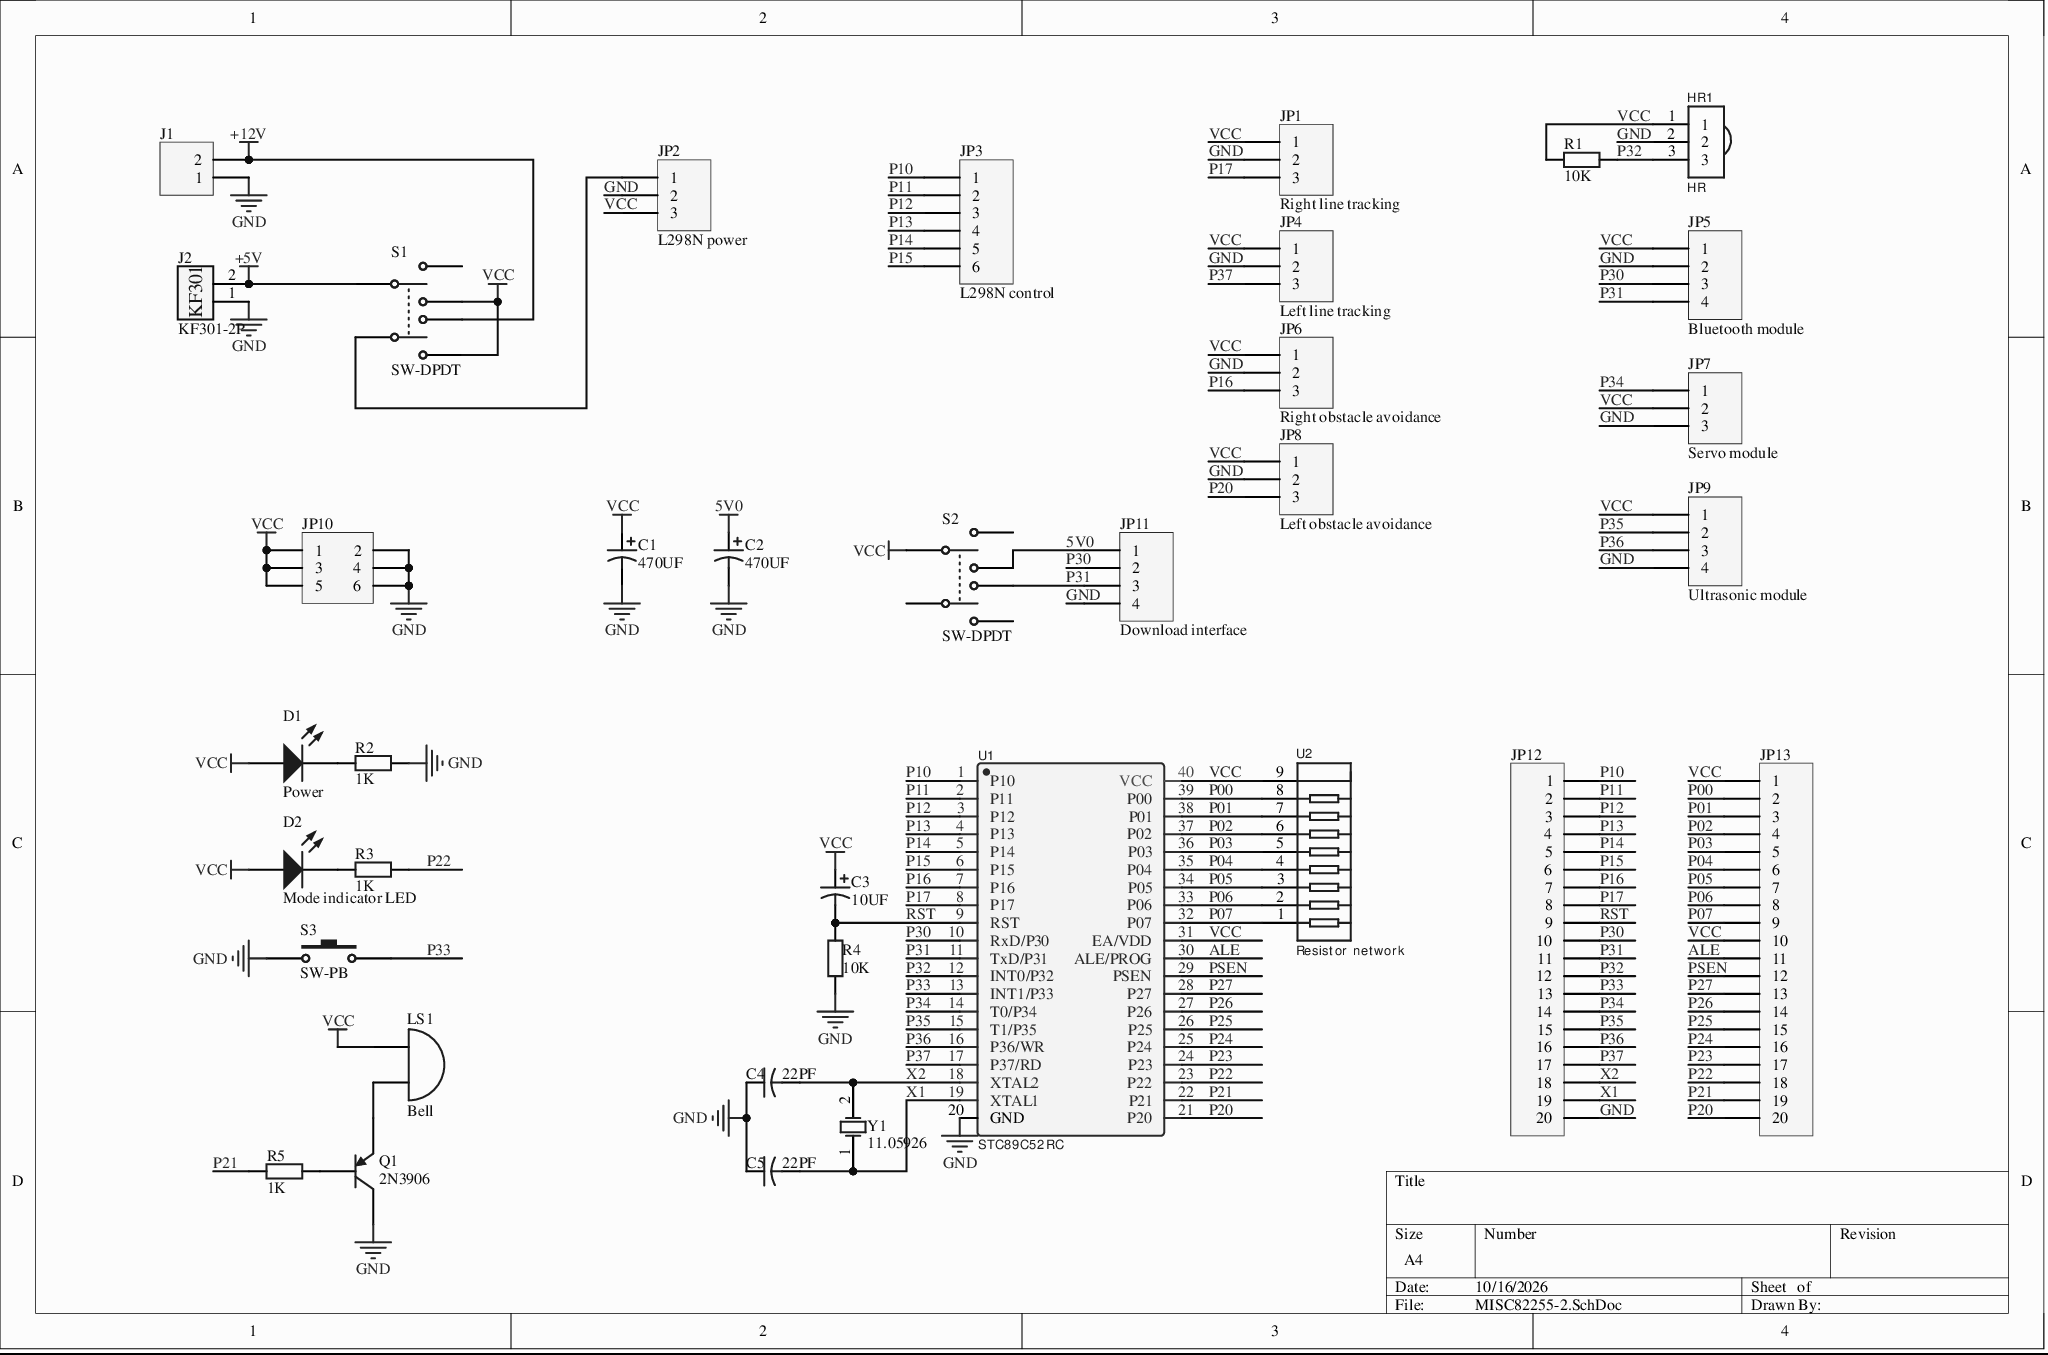
[diagram p0: MISC82255-2.SchDoc]
# Altium project MISC82255-5.PrjPcb
1 sheet, 36 parts. Net scope: global (net labels, ports and power ports of the same name join across sheets).
Board file: MISC82255.PcbDoc

## Sheet MISC82255-2.SchDoc
size A4

### Parts
C1  470UF  [DR]
C2  470UF  [DR]
C3  10UF  [DR]
C4  22PF  [CAPR5-4X5]
C5  22PF  [CAPR5-4X5]
D1  Power  [LED-1]
D2  Mode indicator LED  [LED-1]
HR1  HR  [SIP3]
J1  Header 2  [HDR1X2]  (value not drawn)
J2  KF301-2P  [KF301-5.0-2P]
JP1  Right line tracking  [HDR1X3]
JP2  L298N power  [HDR1X3]
JP3  L298N control  [HDR1X6]
JP4  Left line tracking  [HDR1X3]
JP5  Bluetooth module  [HDR1X4]
JP6  Right obstacle avoidance  [HDR1X3]
JP7  Servo module  [HDR1X3]
JP8  Left obstacle avoidance  [HDR1X3]
JP9  Ultrasonic module  [HDR1X4]
JP10  Header 3X2  [HDR2X3]  (value not drawn)
JP11  Download interface  [HDR1X4]
JP12  Header 20  [HDR1X20]  (value not drawn)
JP13  Header 20  [HDR1X20]  (value not drawn)
LS1  Bell  [PIN2]
Q1  2N3906  [TO-92A]
R1  10K  [AXIAL-0.4]
R2  1K  [AXIAL-0.4]
R3  1K  [AXIAL-0.4]
R4  10K  [AXIAL-0.4]
R5  1K  [AXIAL-0.4]
S1  SW-DPDT  [DPDT-6]
S2  SW-DPDT  [DPDT-6]
S3  SW-PB  [SPST-2]
U1  STC89C52RC  [STC89C52RC]
U2  Resistor network  [paizu]
Y1  11.05926  [R38]

### Nets
5V0: C2.1 JP11.1 S2.3
+5V: J2.2 S1.1
+12V: J1.2 S1.5
GND: C1.2 C2.2 C4.1 C5.1 HR1.2 J1.1 J2.1 JP1.2 JP2.2 JP4.2 JP5.2 JP6.2 JP7.3 JP8.2 JP9.4 JP10.2 JP10.4 JP10.6 JP11.4 JP12.20 Q1.3(C) R2.2 R4.1 S3.1 U1.20(GND)
VCC: C1.1 C3.1 D1.1(A) D2.1(A) HR1.1 JP1.1 JP2.3 JP4.1 JP5.1 JP6.1 JP7.2 JP8.1 JP9.1 JP10.1 JP10.3 JP10.5 JP13.1 JP13.10 LS1.1(A) R1.1 S1.3 S1.6 S2.1 U1.31(EA/VDD) U1.40(VCC) U2.9
ALE: JP13.11 U1.30(ALE/PROG)
P00: JP13.2 U1.39(P00) U2.8
P01: JP13.3 U1.38(P01) U2.7
P02: JP13.4 U1.37(P02) U2.6
P03: JP13.5 U1.36(P03) U2.5
P04: JP13.6 U1.35(P04) U2.4
P05: JP13.7 U1.34(P05) U2.3
P06: JP13.8 U1.33(P06) U2.2
P07: JP13.9 U1.32(P07) U2.1
P10: JP3.1 JP12.1 U1.1(P10)
P11: JP3.2 JP12.2 U1.2(P11)
P12: JP3.3 JP12.3 U1.3(P12)
P13: JP3.4 JP12.4 U1.4(P13)
P14: JP3.5 JP12.5 U1.5(P14)
P15: JP3.6 JP12.6 U1.6(P15)
P16: JP6.3 JP12.7 U1.7(P16)
P17: JP1.3 JP12.8 U1.8(P17)
P20: JP8.3 JP13.20 U1.21(P20)
P21: JP13.19 R5.1 U1.22(P21)
P22: JP13.18 R3.2 U1.23(P22)
P23: JP13.17 U1.24(P23)
P24: JP13.16 U1.25(P24)
P25: JP13.15 U1.26(P25)
P26: JP13.14 U1.27(P26)
P27: JP13.13 U1.28(P27)
P30: JP5.3 JP11.2 JP12.10 U1.10(RxD/P30)
P31: JP5.4 JP11.3 JP12.11 S2.5 U1.11(TxD/P31)
P32: HR1.3 JP12.12 R1.2 U1.12(INT0/P32)
P33: JP12.13 S3.2 U1.13(INT1/P33)
P34: JP7.1 JP12.14 U1.14(T0/P34)
P35: JP9.2 JP12.15 U1.15(T1/P35)
P36: JP9.3 JP12.16 U1.16(P36/WR)
P37: JP4.3 JP12.17 U1.17(P37/RD)
PSEN: JP13.12 U1.29(PSEN)
RST: C3.2 JP12.9 R4.2 U1.9(RST)
X1: C5.2 JP12.19 U1.19(XTAL1) Y1.1(OSC1)
X2: C4.2 JP12.18 U1.18(XTAL2) Y1.2(OSC2)
NetD1_2: D1.2(K) R2.1
NetD2_2: D2.2(K) R3.1
NetJP2_1: JP2.1 S1.4
NetLS1_2: LS1.2(B) Q1.1(E)
NetQ1_2: Q1.2(B) R5.2

Not connected (* = marked no-connect by the designer): S1 2; S2 2 4 6

### Library data of the parts
C1-C3 = Cap Pol1: Polarized Capacitor (Radial); Value: 100pF; Published: 8-Jun-2000; LatestRevisionDate: 17-Jul-2002; LatestRevisionNote: Re-released for DXP Platform.; PackageReference: RB7.6-15; PackageDescription: Polarized Capacitor (Radial); 2 Leads; Publisher: Altium Limited
C4 C5 = Cap2: Capacitor; Value: 100pF; Published: 23-Sep-2002; PackageReference: CAPR5-4X5; PackageDescription: Capacitor; 2 Leads; Publisher: Altium Limited
D1 D2 = LED1: Typical RED GaAs LED; Published: 8-Jun-2000; LatestRevisionDate: 08-Jul-2005; LatestRevisionNote: Mech Layer 1 removed.; PackageReference: LED-1; PackageDescription: LED; 2 Leads; Publisher: Altium Limited
J1 = Header 2: Header, 2-Pin; LatestRevisionDate: 17-Jul-2002; LatestRevisionNote: Re-released for DXP Platform.; Publisher: Altium Limited
JP1 JP2 JP4 JP6-JP8 = Header 3: Header, 3-Pin; LatestRevisionDate: 17-Jul-2002; LatestRevisionNote: Re-released for DXP Platform.; Publisher: Altium Limited
JP3 = Header 6: Header, 6-Pin; LatestRevisionDate: 17-Jul-2002; LatestRevisionNote: Re-released for DXP Platform.; Publisher: Altium Limited
JP5 JP9 JP11 = Header 4: Header, 4-Pin; LatestRevisionDate: 17-Jul-2002; LatestRevisionNote: Re-released for DXP Platform.; Publisher: Altium Limited
JP10 = Header 3X2: Header, 3-Pin, Dual row; LatestRevisionDate: 17-Jul-2002; LatestRevisionNote: Re-released for DXP Platform.; Publisher: Altium Limited
JP12 JP13 = Header 20: Header, 20-Pin; LatestRevisionDate: 17-Jul-2002; LatestRevisionNote: Re-released for DXP Platform.; Publisher: Altium Limited
LS1 = Bell: Electrical Bell; Published: 24-Mar-1999; LatestRevisionDate: 17-Jul-2002; LatestRevisionNote: Re-released for DXP Platform.; PackageReference: PIN2; Publisher: Altium Limited
Q1 = 2N3906: PNP General Purpose Amplifier; Published: 8-Jun-2000; LatestRevisionDate: 15-Jan-2003; LatestRevisionNote: PCB Footprint 'BCY-W3/D4.7' replaced; DatasheetVersion: 1997; PackageVersion: Sep-1998; PackageReference: TO-92A; PackageDescription: TO, Flat Index; 3 In-Line, Axial Leads; Body Dia. 4.5mm; Leads 0.51 x 0.48 mm (max); ComponentLink1Description: Manufacturer Link; ComponentLink2Description: Datasheet; ComponentLink2URL: http://www.fairchildsemi.com/ds/2N%2F2N3906.pdf; Publisher: Altium Limited
R1 R4 = Res2: Resistor; Value: 1K; Published: 8-Jun-2000; LatestRevisionDate: 17-Jul-2002; LatestRevisionNote: Re-released for DXP Platform.; PackageReference: AXIAL-0.4; PackageDescription: Axial Device, Thru-Hole; 2 Leads; 0.4 in Pin Spacing; Publisher: Altium Limited
R2 R3 R5 = Res2: Resistor; Published: 8-Jun-2000; LatestRevisionDate: 17-Jul-2002; LatestRevisionNote: Re-released for DXP Platform.; PackageReference: AXIAL-0.4; PackageDescription: Axial Device, Thru-Hole; 2 Leads; 0.4 in Pin Spacing; Value: 1K; Publisher: Altium Limited
S1 S2 = SW-DPDT: Double-Pole, Double-Throw Switch; Published: 24-Mar-1999; LatestRevisionDate: 17-Jul-2002; LatestRevisionNote: Re-released for DXP Platform.; PackageReference: DPDT-6; PackageDescription: Switch; 6 Leads; Publisher: Altium Limited
S3 = SW-PB: Switch; Published: 24-Mar-1999; LatestRevisionDate: 17-Jul-2002; LatestRevisionNote: Re-released for DXP Platform.; PackageReference: SPST-2; PackageDescription: Switch; 2 Leads; Publisher: Altium Limited
U2 = 排阻
Y1 = XTAL: Crystal Oscillator; Published: 8-Jun-2000; LatestRevisionDate: 17-Jul-2002; LatestRevisionNote: Re-released for DXP Platform.; PackageReference: R38; PackageDescription: Crystal, Thru-Hole; 2 Leads; Body 3.1 x 8.2 mm (Dia.xH); Publisher: Altium Limited